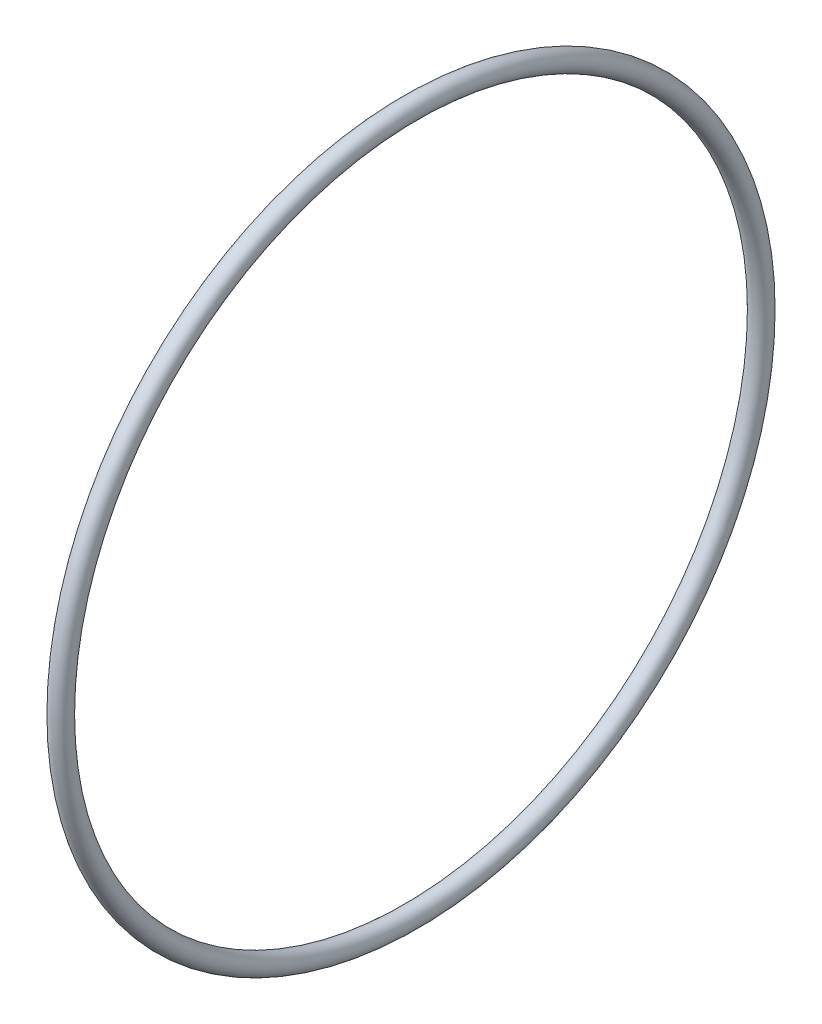
SolidWorks part; units mm, degrees
ref_plane "Front Plane" through (0, 0, 0) normal (0, 0, 1) x (1, 0, 0)
ref_plane "Top Plane" through (0, 0, 0) normal (0, 1, 0) x (1, 0, 0)
ref_plane "Right Plane" through (0, 0, 0) normal (1, 0, 0) x (0, 0, -1)
sketch "Sketch1" plane through (0, 0, 0) normal (0, 0, 1) x (1, 0, 0)
  line L0 (0, 0) -> (5, 0)
  circle A0 centre (5, 47.35) radius 1.325
  dimension "D3" = 2.65
  dimension "D1" = 5
  dimension "D2" = 47.35
revolve "Revolve1" add sketch "Sketch1" angle 360 about L0
